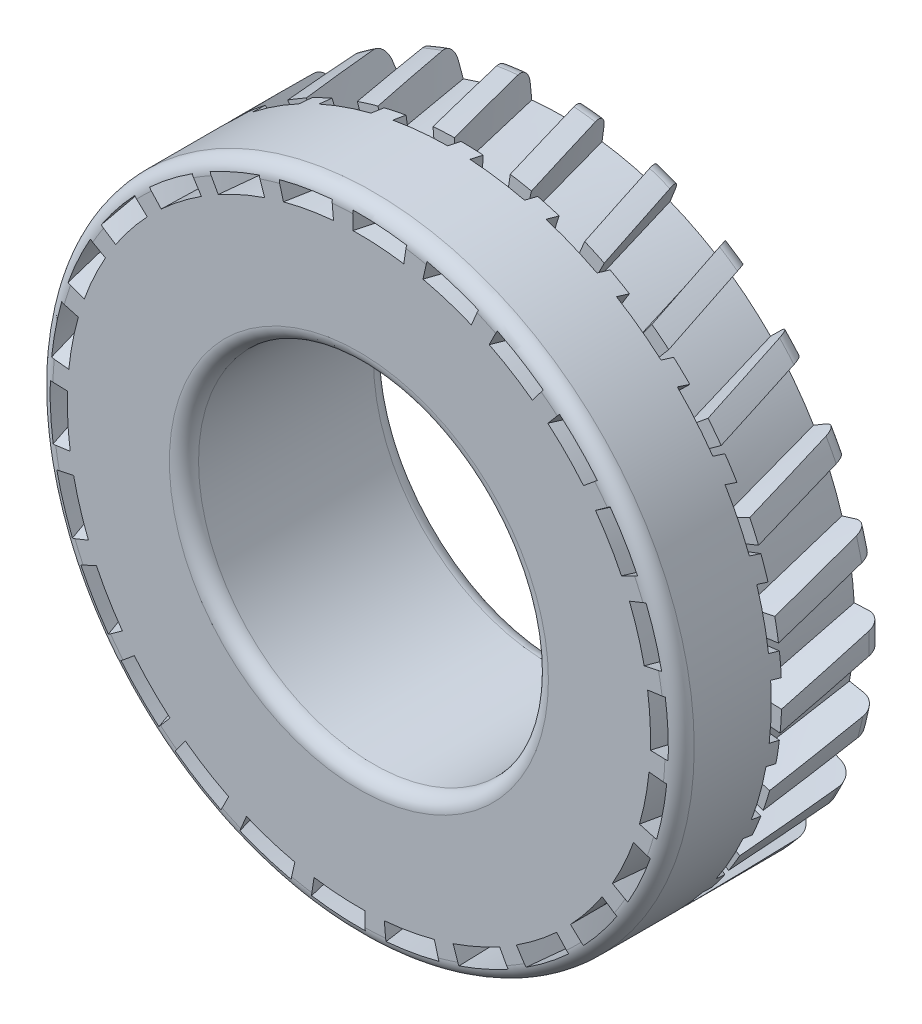
SolidWorks part; units mm, degrees
ref_plane "前视基准面" through (0, 0, 0) normal (0, 0, 1) x (1, 0, 0)
ref_plane "上视基准面" through (0, 0, 0) normal (0, 1, 0) x (1, 0, 0)
ref_plane "右视基准面" through (0, 0, 0) normal (1, 0, 0) x (0, 0, -1)
sketch "草图1" plane through (0, 0, 0) normal (0, 0, 1) x (1, 0, 0)
  circle A0 centre (0, 0) radius 220
  circle A1 centre (0, 0) radius 120
extrude "凸台-拉伸1" add sketch "草图1" along normal mid plane 140
sketch "草图5" plane through (0, 0, 0) normal (0, 0, 1) x (1, 0, 0)
  line L2 (-37.8574, 217.7334) -> (-34.2108, 197.0523)
  line L3 (0, 200) -> (0, 221)
  arc A2 (0, 200) -> (-34.2108, 197.0523) centre (0, 0) ccw
  arc A3 (0, 221) -> (-37.8574, 217.7334) centre (0, 0) ccw
  dimension "D1" = 200
  dimension "D2" = 221
  dimension "D3" = 10
sketch "草图6" plane through (0, 0, 70) normal (0, 0, 1) x (1, 0, 0)
  line L5 (-17.4311, 199.2389) -> (-18.477, 211.1933)
  line L6 (-54.8696, 204.7763) -> (-51.7638, 193.1852)
  arc A2 (-17.4311, 199.2389) -> (-51.7638, 193.1852) centre (0, 0) ccw
  arc A3 (-18.477, 211.1933) -> (-54.8696, 204.7763) centre (0, 0) ccw
  dimension "D1" = 400
  dimension "D3" = 10
  dimension "D2" = 424
fillet "圆角5" radius 10 4 edges at (120, 0, -70) (120, 0, 70) (220, 0, -70) (220, 0, 70)
loft "切除-放样3" cut profiles "草图5", "草图6"
pattern_circular "阵列(圆周)1" count 26 over 360 about axis through (0, 0, 70) along (0, 0, 1) of "切除-放样3"
sketch "草图7" plane through (0, 0, 0) normal (0, 0, 1) x (1, 0, 0)
  line L3 (-17.4311, 199.2389) -> (-19.2614, 220.159)
  line L4 (-57.199, 213.4696) -> (-51.7638, 193.1852)
  arc A2 (-17.4311, 199.2389) -> (-51.7638, 193.1852) centre (0, 0) ccw
  arc A3 (-19.2614, 220.159) -> (-57.199, 213.4696) centre (0, 0) ccw
  dimension "D1" = 200
  dimension "D2" = 221
  dimension "D3" = 10
sketch "草图8" plane through (0, 0, -70) normal (0, 0, -1) x (-1, 0, 0)
  line L2 (38.3762, 217.6425) -> (34.7296, 196.9616)
  line L3 (68.404, 187.9385) -> (75.5865, 207.6721)
  arc A4 (68.404, 187.9385) -> (34.7296, 196.9616) centre (0, 0) ccw
  arc A5 (75.5865, 207.6721) -> (38.3762, 217.6425) centre (0, 0) ccw
  dimension "D1" = 200
  dimension "D2" = 221
  dimension "D3" = 10
loft "切除-放样4" cut profiles "草图8", "草图7"
pattern_circular "阵列(圆周)2" count 26 over 360 about axis through (0, 0, 70) along (0, 0, 1) of "切除-放样4"
ref_plane "基准面1" through (0, -220, 0) normal (0, 1, 0) x (1, 0, 0)
